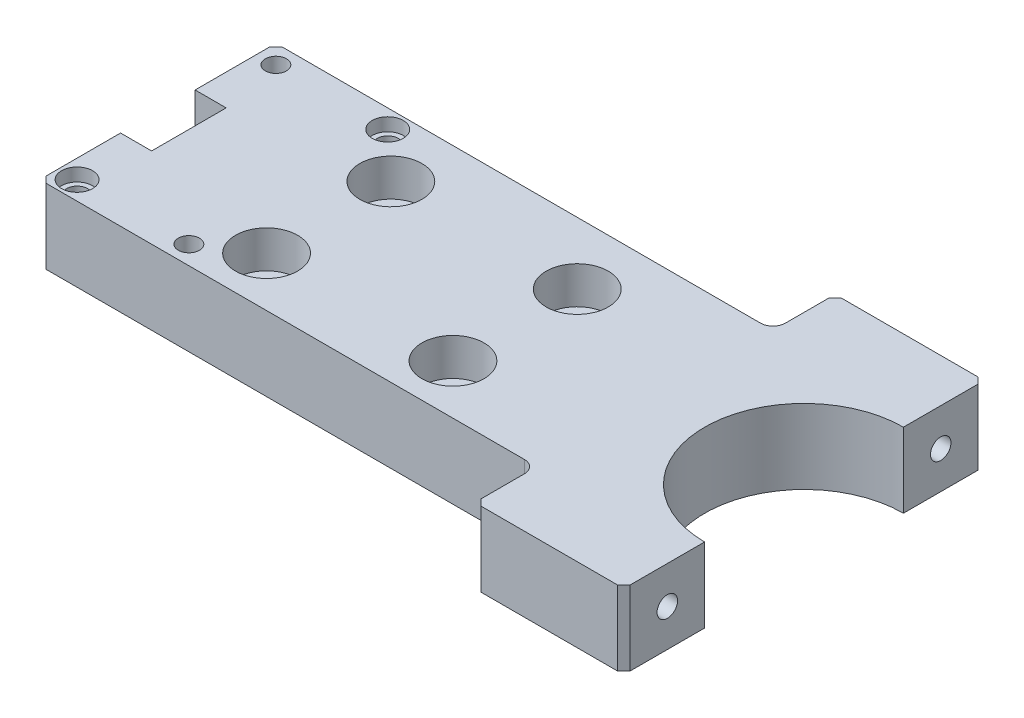
from build123d import *

# Parameters (mm, degrees)
SKETCH1_W                                            = 104
SKETCH1_H                                            = 12
BOSS_EXTRUDE1_DEPTH                                  = 38
SKETCH2_W                                            = 5
SKETCH2_H                                            = 12
CUT_EXTRUDE1_DEPTH                                   = 112.373246339
SKETCH3_R                                            = 16
CUT_EXTRUDE2_DEPTH                                   = 112.373246339
SKETCH4_W                                            = 24
SKETCH4_H                                            = 12
BOSS_EXTRUDE2_DEPTH                                  = 10
SKETCH5_W                                            = 24
SKETCH5_H                                            = 12
BOSS_EXTRUDE3_DEPTH                                  = 10
CHAMFER1_SIZE                                        = 1
FILLET1_R                                            = 2
HOLE_SIZE_PER_SOCKET_HEAD_CAP_SCREW_TYPE_D           = 3.4
HOLE_SIZE_PER_SOCKET_HEAD_CAP_SCREW_TYPE_CBORE_D     = 5.5
HOLE_SIZE_PER_SOCKET_HEAD_CAP_SCREW_TYPE_CBORE_DEPTH = 4
SKETCH8_R                                            = 2.5
CUT_EXTRUDE3_DEPTH                                   = 2.1
HOLE_SIZE_PER_SOCKET_HEAD_CAP_SCREW_2_D              = 5.5
HOLE_SIZE_PER_SOCKET_HEAD_CAP_SCREW_2_CBORE_D        = 10
HOLE_SIZE_PER_SOCKET_HEAD_CAP_SCREW_2_CBORE_DEPTH    = 6
SKETCH11_R                                           = 4.5
CUT_EXTRUDE4_DEPTH                                   = 2.1
M4_TAPPED_HOLE1_D                                    = 3.3
M4_TAPPED_HOLE1_DEPTH                                = 11.5
M4_TAPPED_HOLE1_TIP                                  = 0.991420021


with BuildPart() as part:
    # Sketch1 → Boss-Extrude1 (new body)
    with BuildSketch(Plane.XY):
        with Locations((52, 6)):
            Rectangle(SKETCH1_W, SKETCH1_H)
    extrude(amount=BOSS_EXTRUDE1_DEPTH)

    # Sketch2 → Cut-Extrude1 (cut, through all)
    with BuildSketch(Plane(origin=(0, 12, 0), x_dir=(1, 0, 0), z_dir=(0, 1, 0))):
        with Locations((2.5, -19)):
            Rectangle(SKETCH2_W, SKETCH2_H)
    extrude(amount=-CUT_EXTRUDE1_DEPTH, mode=Mode.SUBTRACT)

    # Sketch3 → Cut-Extrude2 (cut, through all)
    with BuildSketch(Plane(origin=(0, 12, 0), x_dir=(1, 0, 0), z_dir=(0, 1, 0))):
        with Locations((104, -19)):
            Circle(SKETCH3_R)
    extrude(amount=-CUT_EXTRUDE2_DEPTH, mode=Mode.SUBTRACT)

    # Sketch4 → Boss-Extrude2 (add)
    with BuildSketch(Plane(origin=(0, 0, 0), x_dir=(-1, 0, 0), z_dir=(0, 0, -1))):
        with Locations((-92, 6)):
            Rectangle(SKETCH4_W, SKETCH4_H)
    extrude(amount=BOSS_EXTRUDE2_DEPTH)

    # Sketch5 → Boss-Extrude3 (add)
    with BuildSketch(Plane.XY.offset(38)):
        with Locations((92, 6)):
            Rectangle(SKETCH5_W, SKETCH5_H)
    extrude(amount=BOSS_EXTRUDE3_DEPTH)

    # Chamfer1
    chamfer1_edges = [part.edges().sort_by_distance(p)[0] for p in [
        (0, 6, 0),
        (0, 6, 38),
        (104, 6, 48),
        (80, 6, 48),
        (104, 6, -10),
        (80, 6, -10),
    ]]
    chamfer(chamfer1_edges, length=CHAMFER1_SIZE)

    # Fillet1
    fillet1_edges = [part.edges().sort_by_distance(p)[0] for p in [
        (80, 6, 38),
        (80, 6, 0),
    ]]
    fillet(fillet1_edges, radius=FILLET1_R)

    # Hole size per socket head cap screw type (through all)
    with Locations(Plane(origin=(0, 0, 0), x_dir=(-1, 0, 0), z_dir=(0, -1, 0))):
        with Locations((-3, -35), (-21, -3), (-3, -3), (-21, -35)):
            CounterBoreHole(HOLE_SIZE_PER_SOCKET_HEAD_CAP_SCREW_TYPE_D / 2, HOLE_SIZE_PER_SOCKET_HEAD_CAP_SCREW_TYPE_CBORE_D / 2, HOLE_SIZE_PER_SOCKET_HEAD_CAP_SCREW_TYPE_CBORE_DEPTH)

    # Sketch8 → Cut-Extrude3 (cut)
    with BuildSketch(Plane(origin=(0, 12, 0), x_dir=(1, 0, 0), z_dir=(0, 1, 0))):
        with Locations(Location((3, -35, 0), (0, 0, 270))):
            Circle(SKETCH8_R)
        with Locations(Location((21, -3, 0), (0, 0, 270))):
            Circle(SKETCH8_R)
    extrude(amount=-CUT_EXTRUDE3_DEPTH, mode=Mode.SUBTRACT)

    # Hole size per socket head cap screw  2 (through all)
    with Locations(Plane(origin=(0, 12, 0), x_dir=(1, 0, 0), z_dir=(0, 1, 0))):
        with Locations((28.5, -10), (28.5, -30), (58.5, -10), (58.5, -30)):
            CounterBoreHole(HOLE_SIZE_PER_SOCKET_HEAD_CAP_SCREW_2_D / 2, HOLE_SIZE_PER_SOCKET_HEAD_CAP_SCREW_2_CBORE_D / 2, HOLE_SIZE_PER_SOCKET_HEAD_CAP_SCREW_2_CBORE_DEPTH)

    # Sketch11 → Cut-Extrude4 (cut)
    with BuildSketch(Plane.XZ):
        with Locations(Location((28.5, 30, 0), (0, 0, 270))):
            Circle(SKETCH11_R)
        with Locations(Location((58.5, 10, 0), (0, 0, 270))):
            Circle(SKETCH11_R)
    extrude(amount=-CUT_EXTRUDE4_DEPTH, mode=Mode.SUBTRACT)

    # M4 Tapped Hole1
    with Locations(Plane(origin=(104, 0, 0), x_dir=(0, 0, -1), z_dir=(1, 0, 0))):
        with Locations((3, 6), (-41, 6)):
            Hole(M4_TAPPED_HOLE1_D / 2, depth=M4_TAPPED_HOLE1_DEPTH)
            with Locations((0, 0, -(M4_TAPPED_HOLE1_DEPTH + M4_TAPPED_HOLE1_TIP / 2))):  # 118° drill point
                Cone(0, M4_TAPPED_HOLE1_D / 2, M4_TAPPED_HOLE1_TIP, mode=Mode.SUBTRACT)


solid = part.part
